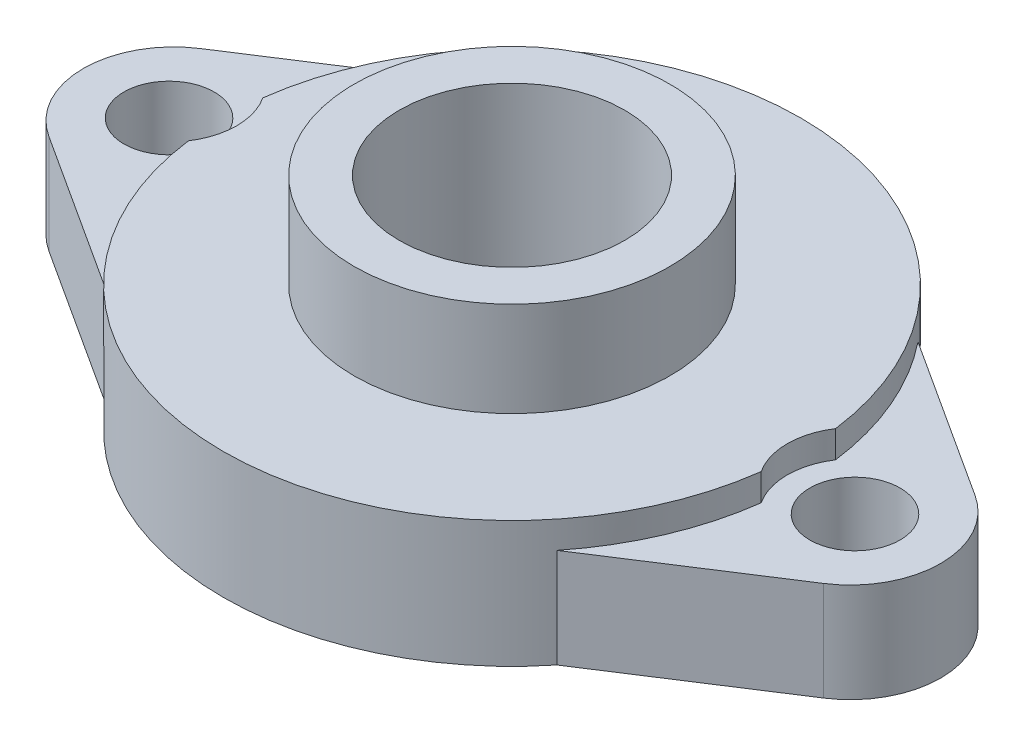
from build123d import *

# Parameters (mm, degrees)
SKETCH_1_R          = 32
EXTRUDE_1_DEPTH     = 14
EXTRUDE_2_DEPTH     = 11
SKETCH_3_R          = 5
CUT_EXTRUDE_1_DEPTH = 59.959732021
SKETCH_4_R          = 7.5
CUT_EXTRUDE_2_DEPTH = 3
SKETCH_5_R          = 17.5
EXTRUDE_3_DEPTH     = 24.5
SKETCH_6_R          = 20
CUT_EXTRUDE_3_DEPTH = 7
EXTRUDE_START       = 3.5
SKETCH_7_R          = 17.5
EXTRUDE_4_DEPTH     = 3.5
SKETCH_8_R          = 12.5
CUT_EXTRUDE_4_DEPTH = 63.293659388


with BuildPart() as part:
    # 草图1 → 凸台-拉伸1 (new body)
    with BuildSketch(Plane(origin=(0, 0, 0), x_dir=(1, 0, 0), z_dir=(0, 1, 0))):
        with Locations(Location((0, 0, 0), (0, 0, 270))):
            Circle(SKETCH_1_R)
    extrude(amount=EXTRUDE_1_DEPTH)

    # 草图2 → 凸台-拉伸2 (add)
    with BuildSketch(Plane(origin=(0, 0, 0), x_dir=(1, 0, 0), z_dir=(0, 1, 0))):
        with BuildLine():
            Line((42.928542082, 8.398269516), (24.979991994, 20))
            ThreePointArc((24.979991994, 20), (32, 0), (24.979991994, -20))
            Line((24.979991994, -20), (42.928542082, -8.398269516))
            ThreePointArc((42.928542082, -8.398269516), (47.5, 0), (42.928542082, 8.398269516))
        make_face()
    extrude_2 = extrude(amount=EXTRUDE_2_DEPTH)

    # 镜向1: 凸台-拉伸2 across plane
    add(extrude_2.mirror(Plane(origin=(0, 0, 0), x_dir=(0, 0, 1), z_dir=(1, 0, 0))))

    # 草图3 → 切除-拉伸1 (cut, through all)
    with BuildSketch(Plane(origin=(0, 0, 0), x_dir=(1, 0, 0), z_dir=(0, 1, 0))):
        with Locations(Location((-38, 0, 0), (0, 0, 270))):
            Circle(SKETCH_3_R)
        with Locations(Location((38, 0, 0), (0, 0, 270))):
            Circle(SKETCH_3_R)
    extrude(amount=CUT_EXTRUDE_1_DEPTH, mode=Mode.SUBTRACT)

    # 草图4 → 切除-拉伸2 (cut)
    with BuildSketch(Plane(origin=(0, 14, 0), x_dir=(1, 0, 0), z_dir=(0, 1, 0))):
        with Locations((-38, 0)):
            Circle(SKETCH_4_R)
        with Locations((38, 0)):
            Circle(SKETCH_4_R)
    extrude(amount=-CUT_EXTRUDE_2_DEPTH, mode=Mode.SUBTRACT)

    # 草图5 → 凸台-拉伸3 (add)
    with BuildSketch(Plane(origin=(0, 0, 0), x_dir=(1, 0, 0), z_dir=(0, 1, 0))):
        with Locations(Location((0, 0, 0), (0, 0, 270))):
            Circle(SKETCH_5_R)
    extrude(amount=EXTRUDE_3_DEPTH)

    # 草图6 → 切除-拉伸3 (cut)
    with BuildSketch(Plane.XZ):
        with Locations(Location((0, 0, 0), (0, 0, 270))):
            Circle(SKETCH_6_R)
    extrude(amount=-CUT_EXTRUDE_3_DEPTH, mode=Mode.SUBTRACT)

    # 草图7 → 凸台-拉伸4 (add)
    with BuildSketch(Plane.XZ.offset(-7).offset(EXTRUDE_START)):
        with Locations(Location((0, 0, 0), (0, 0, 90))):
            Circle(SKETCH_7_R)
    extrude(amount=-EXTRUDE_4_DEPTH)

    # 草图8 → 切除-拉伸4 (cut, through all)
    with BuildSketch(Plane(origin=(0, 24.5, 0), x_dir=(1, 0, 0), z_dir=(0, 1, 0))):
        with Locations(Location((0, 0, 0), (0, 0, 270))):
            Circle(SKETCH_8_R)
    extrude(amount=-CUT_EXTRUDE_4_DEPTH, mode=Mode.SUBTRACT)


solid = part.part
